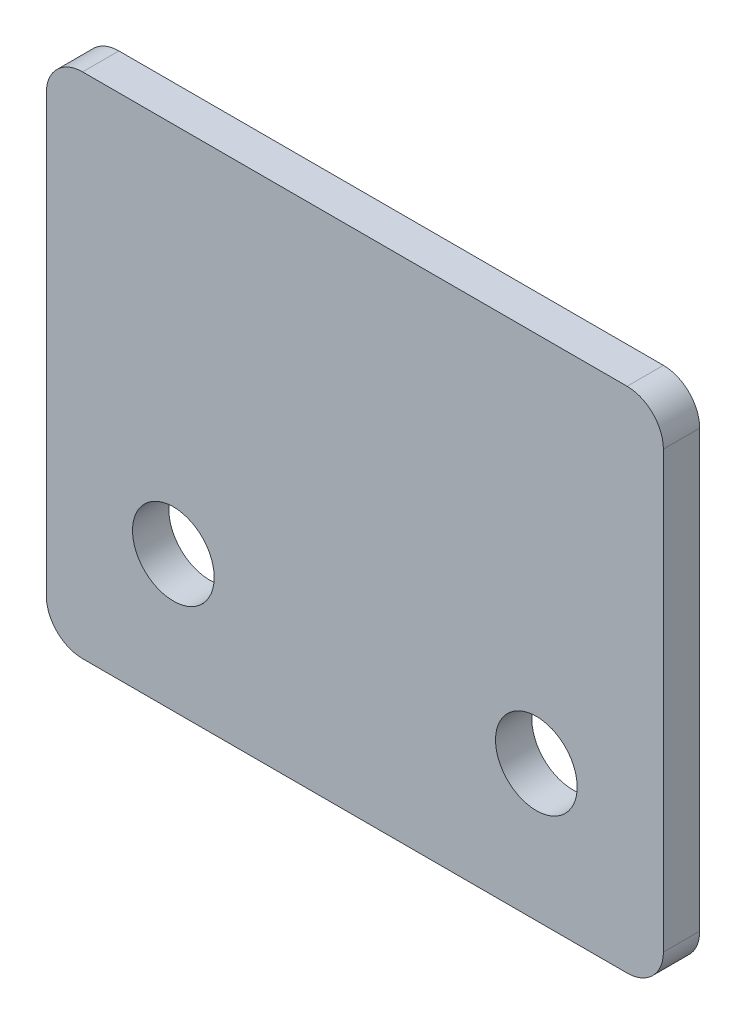
SolidWorks part; units mm, degrees
material "SUS304"
ref_plane "Front Plane" through (0, 0, 0) normal (0, 0, 1) x (1, 0, 0)
ref_plane "Top Plane" through (0, 0, 0) normal (0, 1, 0) x (1, 0, 0)
ref_plane "Right Plane" through (0, 0, 0) normal (1, 0, 0) x (0, 0, -1)
sketch "Sketch1" plane through (0, 0, 0) normal (0, 0, 1) x (1, 0, 0)
  line L0 (0, 0) -> (0, 28) construction
  line L1 (17, 0) -> (-17, 0)
  line L2 (17, 0) -> (17, 28)
  line L3 (17, 28) -> (-17, 28)
  line L4 (-17, 0) -> (-17, 28)
  circle A0 centre (-10, 7.5) radius 2.25
  circle A1 centre (10, 7.5) radius 2.25
  dimension "D3" = 4.5
  dimension "D4" = 7.5
  dimension "D5" = 20
  dimension "D1" = 34
  dimension "D2" = 28
extrude "Boss-Extrude1" add sketch "Sketch1" along normal blind 2
fillet "Fillet1" radius 2 4 edges at (-17, 28, 1) (17, 28, 1) (-17, 0, 1) (17, 0, 1)
